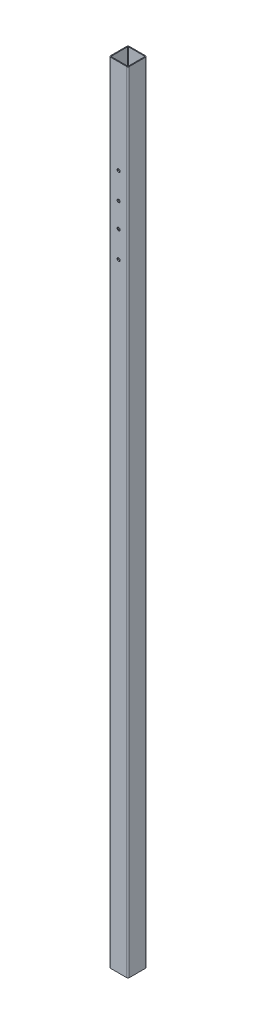
SolidWorks part; units mm, degrees
ref_plane "Front" through (0, 0, 0) normal (0, 0, 1) x (1, 0, 0)
ref_plane "Top" through (0, 0, 0) normal (0, 1, 0) x (1, 0, 0)
ref_plane "Right" through (0, 0, 0) normal (1, 0, 0) x (0, 0, -1)
sketch "Sketch1" plane through (0, 0, 0) normal (0, 1, 0) x (1, 0, 0)
  line L0 (-21.55, -22.7) -> (21.55, -22.7)
  line L1 (-21.55, -25) -> (21.55, -25)
  line L2 (-25, -21.55) -> (-25, 21.55)
  line L3 (-21.55, 25) -> (21.55, 25)
  line L4 (25, -21.55) -> (25, 21.55)
  line L5 (-25, -25) -> (25, 25) construction
  line L6 (-25, 25) -> (25, -25) construction
  line L7 (22.7, -21.55) -> (22.7, 21.55)
  line L8 (-21.55, 22.7) -> (21.55, 22.7)
  line L9 (-22.7, -21.55) -> (-22.7, 21.55)
  arc A0 (21.55, 25) -> (25, 21.55) centre (21.55, 21.55) cw
  arc A1 (-21.55, -25) -> (-25, -21.55) centre (-21.55, -21.55) cw
  arc A2 (21.55, -25) -> (25, -21.55) centre (21.55, -21.55) ccw
  arc A3 (-25, 21.55) -> (-21.55, 25) centre (-21.55, 21.55) cw
  arc A4 (21.55, -22.7) -> (22.7, -21.55) centre (21.55, -21.55) ccw
  arc A5 (21.55, 22.7) -> (22.7, 21.55) centre (21.55, 21.55) cw
  arc A6 (-22.7, 21.55) -> (-21.55, 22.7) centre (-21.55, 21.55) cw
  arc A7 (-21.55, -22.7) -> (-22.7, -21.55) centre (-21.55, -21.55) cw
  point P0 (0, 0)
  dimension "D3" = 3.45
  dimension "D1" = 50
  dimension "D2" = 50
  dimension "D4" = 2.3
extrude "Boss-Extrude1" add sketch "Sketch1" along normal blind 2097
sketch "Sketch2" plane through (0, 0, -25) normal (0, 0, -1) x (-1, 0, 0)
  line L0 (-21.55, 2097) -> (21.55, 2097) construction
  circle A0 centre (0, 1847) radius 4
  circle A1 centre (0, 1777) radius 4
  circle A2 centre (0, 1712) radius 4
  circle A3 centre (0, 1642) radius 4
  dimension "D1" = 8
  dimension "D5" = 250
  dimension "D2" = 70
  dimension "D3" = 65
  dimension "D4" = 70
extrude "Cut-Extrude1" cut sketch "Sketch2" against normal through all both and the other way through all
